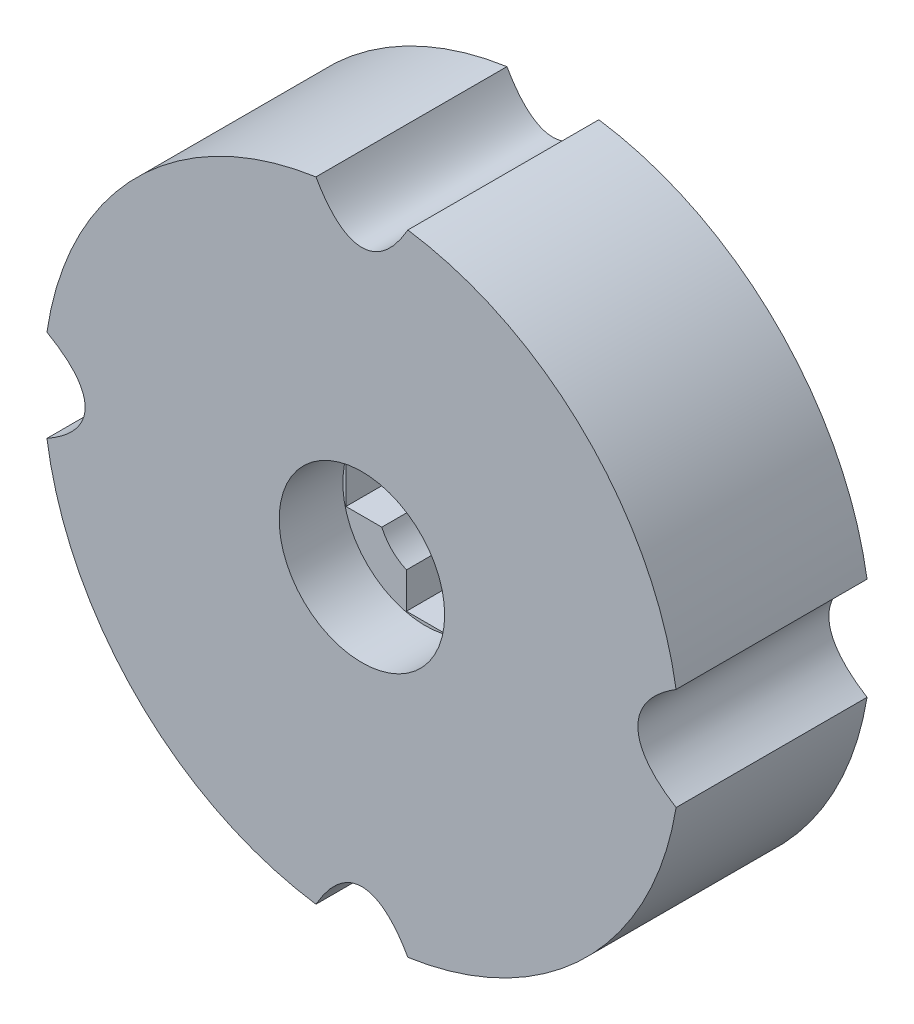
SolidWorks part; units mm, degrees
ref_plane "前视基准面" through (0, 0, 0) normal (0, 0, 1) x (1, 0, 0)
ref_plane "上视基准面" through (0, 0, 0) normal (0, 1, 0) x (1, 0, 0)
ref_plane "右视基准面" through (0, 0, 0) normal (1, 0, 0) x (0, 0, -1)
sketch "草图1" plane through (0, 0, 0) normal (0, 0, 1) x (1, 0, 0)
  line L0 (0, 205.1507) -> (0, -184.8307) construction
  line L1 (-235.3614, 0) -> (151.4491, 0) construction
  line L2 (3, -6.8739) -> (3, -12.5)
  line L3 (-3, 12.5) -> (3, 12.5)
  line L4 (-3, 12.5) -> (-3, 6.8739)
  line L5 (-3, -12.5) -> (3, -12.5)
  line L6 (3, 12.5) -> (3, 6.8739)
  line L7 (-12.5, -3) -> (-6.8739, -3)
  line L8 (-12.5, -3) -> (-12.5, 3)
  line L9 (-12.5, 3) -> (-6.8739, 3)
  line L10 (12.5, -3) -> (12.5, 3)
  line L11 (-3, -6.8739) -> (-3, -12.5)
  line L12 (6.8739, 3) -> (12.5, 3)
  line L13 (6.8739, -3) -> (12.5, -3)
  arc A0 (-7.2209, 49.4758) -> (-49.4758, 7.2212) centre (0, 0) ccw
  arc A1 (-3, 6.8739) -> (-6.8739, 3) centre (0, 0) ccw
  arc A2 (-6.8739, -3) -> (-3, -6.8739) centre (0, 0) ccw
  arc A3 (6.8739, 3) -> (3, 6.8739) centre (0, 0) ccw
  arc A4 (49.3506, 8.0321) -> (7.2209, 49.4758) centre (0, 0) ccw
  arc A5 (7.2209, -49.4758) -> (49.3506, -8.0321) centre (0, 0) ccw
  arc A6 (-49.4758, -7.2212) -> (-7.2209, -49.4758) centre (0, 0) ccw
  arc A7 (3, -6.8739) -> (6.8739, -3) centre (0, 0) ccw
  ellipse E0 centre (0, 97.4624) end of major axis (0, 151.4491) minor radius 15.76 (-7.2209, 49.4758) -> (7.2209, 49.4758) ccw
  ellipse E2 centre (86.3291, 0) end of major axis (43.3506, 0) minor radius 15.7607 (49.3506, 8.0321) -> (49.3506, -8.0321) ccw
  ellipse E3 centre (0, -97.4624) end of major axis (0, -151.4491) minor radius 15.76 (7.2209, -49.4758) -> (-7.2209, -49.4758) ccw
  ellipse E4 centre (-97.4624, 0) end of major axis (-151.4491, 0) minor radius 15.7607 (-49.4758, -7.2212) -> (-49.4758, 7.2212) ccw
  point P1 (48.9585, 12.5)
  point P25 (49.4729, 6.8739)
  dimension "D1" = 100
  dimension "D2" = 25
  dimension "D3" = 12.5
  dimension "D4" = 25
  dimension "D5" = 12.5
  dimension "D6" = 6
  dimension "D7" = 3
  dimension "D8" = 3
  dimension "D9" = 6
  dimension "D10" = 6
  dimension "D11" = 6
  dimension "D12" = 6
  dimension "D13" = 6
  dimension "D14" = 151.4491
  dimension "D15" = 151.4491
  dimension "D16" = 15.7607
  dimension "D17" = 15.7607
  dimension "D18" = 86.3291
  dimension "D19" = 15.76
extrude "拉伸1" add sketch "草图1" along normal mid plane 30
sketch "草图2" plane through (0, 0, 15) normal (0, 0, 1) x (1, 0, 0)
  circle A0 centre (0, 0) radius 13
extrude "拉伸2" cut sketch "草图2" against normal blind 10
